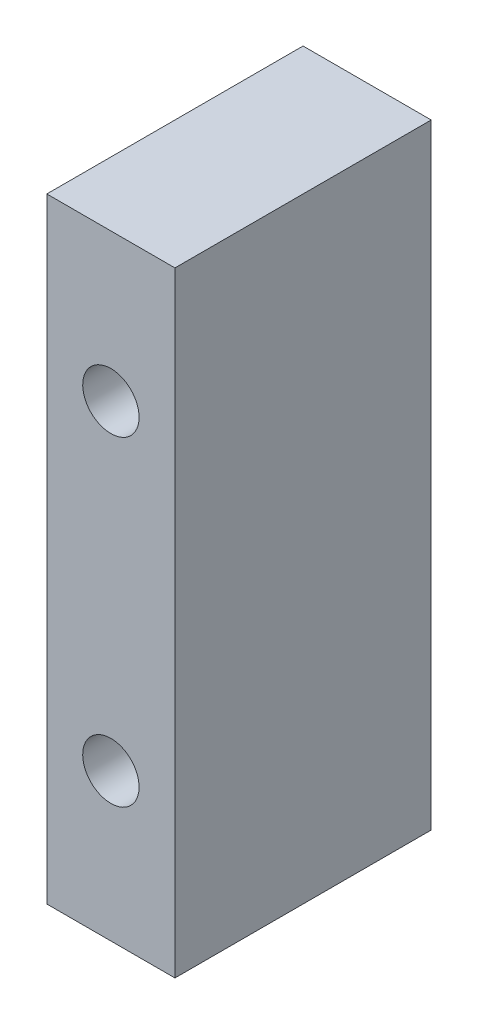
SolidWorks part; units mm, degrees
material "6061铝"
ref_plane "前视基准面" through (0, 0, 0) normal (0, 0, 1) x (1, 0, 0)
ref_plane "上视基准面" through (0, 0, 0) normal (0, 1, 0) x (1, 0, 0)
ref_plane "右视基准面" through (0, 0, 0) normal (1, 0, 0) x (0, 0, -1)
sketch "草图1" plane through (0, 0, 0) normal (1, 0, 0) x (0, 0, -1)
  line L1 (-10, 24) -> (10, 24)
  line L2 (-10, 24) -> (-10, -24)
  line L3 (-10, -24) -> (10, -24)
  line L4 (10, 24) -> (10, -24)
  line L5 (-10, 24) -> (10, -24) construction
  line L6 (-10, -24) -> (10, 24) construction
  point P0 (0, 0)
  dimension "D1" = 20
  dimension "D2" = 48
extrude "凸台-拉伸1" add sketch "草图1" along normal blind 10
hole_wizard "打孔尺寸(%根据)内六角圆柱头螺钉的类型1" positions "草图6" profile "草图8" counterbore size "M4" standard "GB" end condition through all
sketch "草图6" plane through (0, 0, -10) normal (0, 0, -1) x (-1, 0, 0)
  line L0 (0, 0) -> (-16.1883, 0) construction
  line L2 (0, -24) -> (0, 24) construction
  point P0 (-5, -12.5)
  point P2 (-5, 12.5)
  point P9 (0, 0)
  dimension "D1" = 25
  dimension "D2" = 5
sketch "草图8" plane through (5, -12.5, -10) normal (1, 0, 0) x (0, 1, 0)
  line L0 (0, 0) -> (0, 20)
  line L1 (0, 20) -> (2.2, 20)
  line L3 (2.2, 20) -> (2.2, 5)
  line L4 (2.2, 5) -> (4, 5)
  line L5 (4, 5) -> (4, 0)
  line L7 (4, 0) -> (0, 0)
  line L11 (0, -6.35) -> (0, 107.95) construction
  dimension "通孔孔直径" = 4.4
  dimension "通孔孔深度" = 20
  dimension "柱形沉头孔直径" = 8
  dimension "柱形沉头孔深度" = 5
